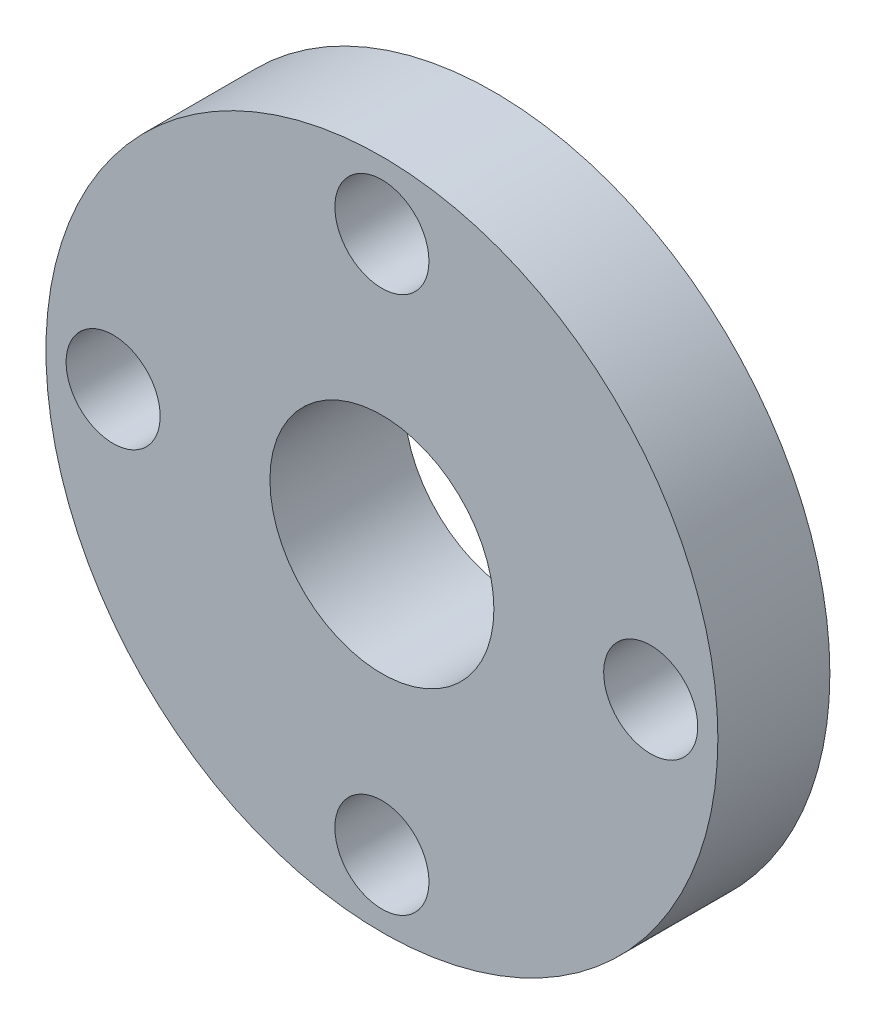
SolidWorks part; units mm, degrees
material "316L"
ref_plane "Front Plane" through (0, 0, 0) normal (0, 0, 1) x (1, 0, 0)
ref_plane "Top Plane" through (0, 0, 0) normal (0, 1, 0) x (1, 0, 0)
ref_plane "Right Plane" through (0, 0, 0) normal (1, 0, 0) x (0, 0, -1)
sketch "Sketch1" plane through (0, 0, 0) normal (0, 0, 1) x (1, 0, 0)
  circle A0 centre (0, 0) radius 15
  dimension "D1" = 30
extrude "Boss-Extrude1" add sketch "Sketch1" along normal blind 5
sketch "Sketch2" plane through (0, 0, 5) normal (0, 0, 1) x (1, 0, 0)
  circle A0 centre (0, 12) radius 2.1
  dimension "D1" = 12
  dimension "D2" = 4.2
extrude "Cut-Extrude1" cut sketch "Sketch2" against normal through all
pattern_circular "CirPattern1" count 4 over 360 about axis through (0, 0, 0) along (0, 0, 1) of "Cut-Extrude1"
sketch "Sketch3" plane through (0, 0, 0) normal (0, 0, -1) x (-1, 0, 0)
  circle A0 centre (0, 0) radius 8
  dimension "D1" = 16
extrude "Boss-Extrude2" add sketch "Sketch3" along normal blind 1
sketch "Sketch4" plane through (0, 0, 5) normal (0, 0, 1) x (1, 0, 0)
  circle A0 centre (0, 0) radius 5
  dimension "D1" = 10
extrude "Cut-Extrude3" cut sketch "Sketch4" against normal through all
chamfer "Chamfer1" [suppressed] distance 1.5 angle 45
